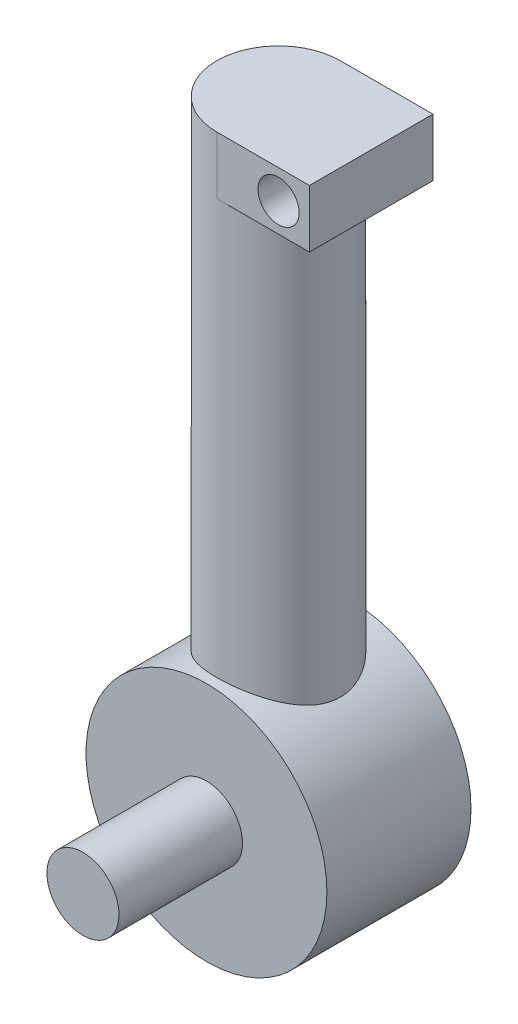
SolidWorks part; units mm, degrees
ref_plane "Front Plane" through (0, 0, 0) normal (0, 0, 1) x (1, 0, 0)
ref_plane "Top Plane" through (0, 0, 0) normal (0, 1, 0) x (1, 0, 0)
ref_plane "Right Plane" through (0, 0, 0) normal (1, 0, 0) x (0, 0, -1)
sketch "Sketch1" plane through (0, 0, 0) normal (0, 0, 1) x (1, 0, 0)
  circle A0 centre (0, 0) radius 58.5
  dimension "D1" = 117
extrude "Boss-Extrude1" add sketch "Sketch1" along normal blind 70
sketch "Sketch2" plane through (0, 0, 0) normal (0, 1, 0) x (1, 0, 0)
  circle A0 centre (0, -35) radius 30
  dimension "D1" = 60
extrude "Boss-Extrude2" add sketch "Sketch2" along normal blind 260
sketch "Sketch4" plane through (0, 260, 0) normal (0, 1, 0) x (1, 0, 0)
  line L0 (0, -65) -> (45, -65)
  line L1 (45, -65) -> (45, -5)
  line L2 (0, -5) -> (45, -5)
  arc A0 (0, -5) -> (0, -65) centre (0, -35) ccw
  circle A1 centre (0, -35) radius 30 construction
  dimension "D2" = 30
  dimension "D1" = 45
extrude "Boss-Extrude4" add sketch "Sketch4" along normal blind 28
sketch "Sketch7" plane through (0, 0, 70) normal (0, 0, 1) x (1, 0, 0)
  circle A0 centre (0, 0) radius 17.5
  dimension "D1" = 35
extrude "Boss-Extrude6" add sketch "Sketch7" along normal blind 60
sketch "Sketch8" plane through (0, 0, 5) normal (0, 0, -1) x (-1, 0, 0)
  line L0 (-45, 288) -> (-45, 260) construction
  circle A0 centre (-30, 274) radius 10
  dimension "D1" = 20
  dimension "D2" = 15
extrude "Cut-Extrude1" cut sketch "Sketch8" against normal through all
